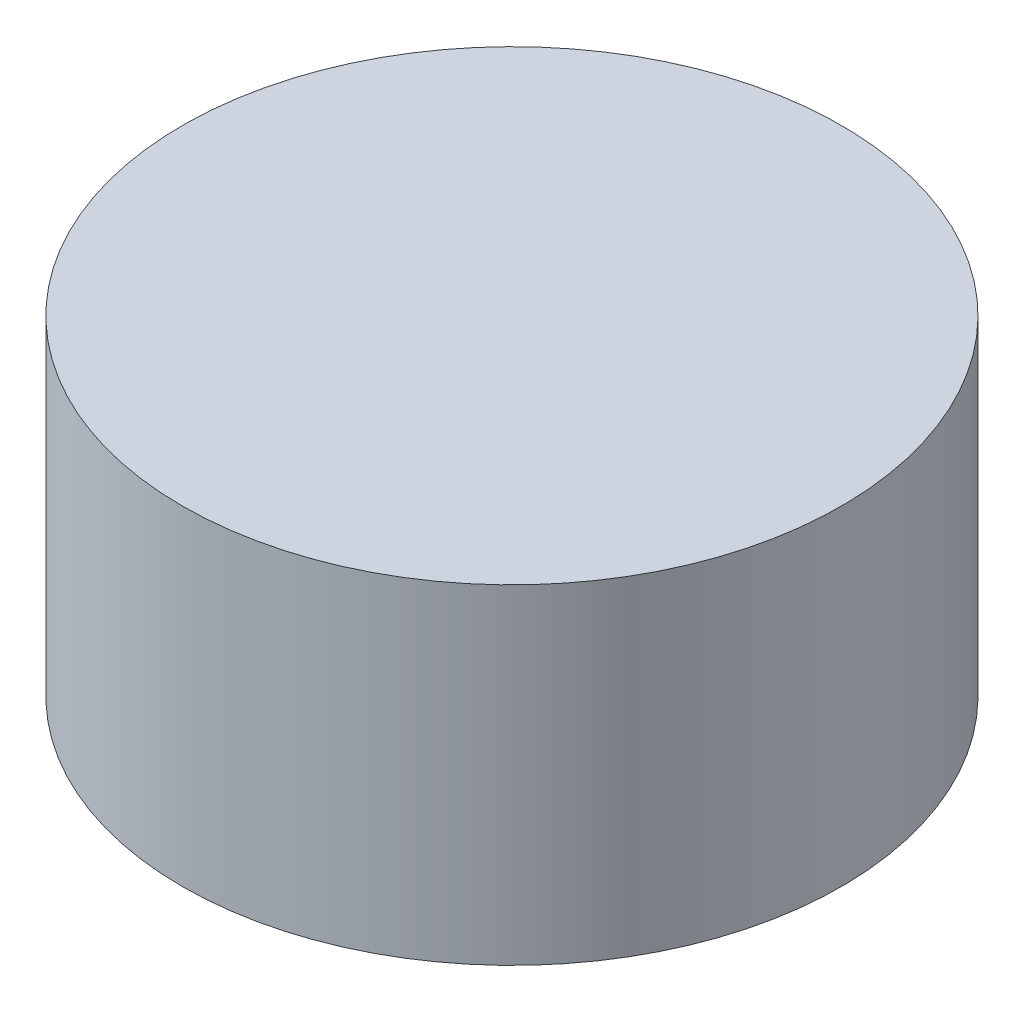
from build123d import *

# Parameters (mm, degrees)
SKETCH1_R           = 5
BOSS_EXTRUDE1_DEPTH = 5


with BuildPart() as part:
    # Sketch1 → Boss-Extrude1 (new body)
    with BuildSketch(Plane(origin=(0, 0, 0), x_dir=(1, 0, 0), z_dir=(0, 1, 0))):
        with Locations(Location((0, 0, 0), (0, 0, 270))):
            Circle(SKETCH1_R)
    extrude(amount=BOSS_EXTRUDE1_DEPTH)


solid = part.part
